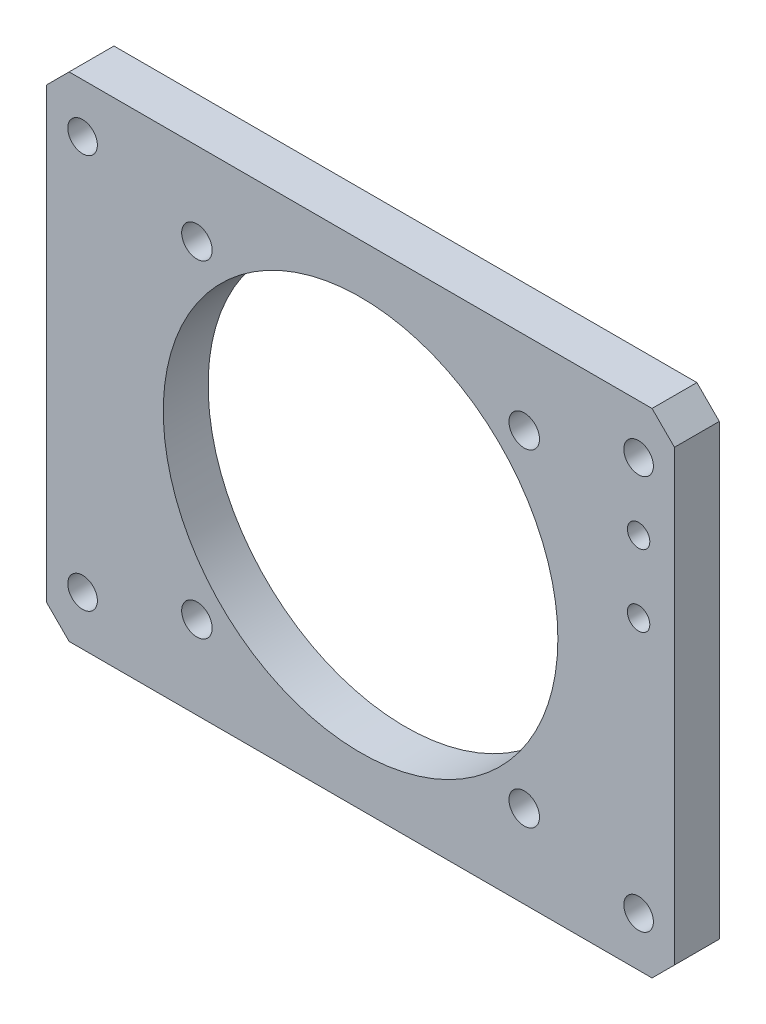
SolidWorks part; units mm, degrees
material "Q235-A"
ref_plane "Front Plane" through (0, 0, 0) normal (0, 0, 1) x (1, 0, 0)
ref_plane "Top Plane" through (0, 0, 0) normal (0, 1, 0) x (1, 0, 0)
ref_plane "Right Plane" through (0, 0, 0) normal (1, 0, 0) x (0, 0, -1)
sketch "Sketch1" plane through (0, 0, 0) normal (0, 0, 1) x (1, 0, 0)
  line L0 (5.5346, 71.5113) -> (5.5346, -38.4887) construction
  line L1 (-64.4654, 71.5113) -> (75.5346, 71.5113)
  line L2 (-64.4654, 71.5113) -> (-64.4654, -38.4887)
  line L3 (-64.4654, -38.4887) -> (75.5346, -38.4887)
  line L4 (75.5346, 71.5113) -> (75.5346, -38.4887)
  line L5 (-64.4654, 16.5113) -> (75.5346, 16.5113) construction
  line L7 (-56.4654, -27.4887) -> (67.5346, -27.4887) construction
  line L8 (-56.4654, -27.4887) -> (-56.4654, 60.5113) construction
  line L9 (-56.4654, 60.5113) -> (67.5346, 60.5113) construction
  line L10 (67.5346, -27.4887) -> (67.5346, 60.5113) construction
  line L11 (-56.4654, -27.4887) -> (67.5346, 60.5113) construction
  line L12 (-56.4654, 60.5113) -> (67.5346, -27.4887) construction
  circle A0 centre (5.5346, 16.5113) radius 44
  circle A1 centre (-56.4654, 60.5113) radius 3.3
  circle A2 centre (-56.4654, -27.4887) radius 3.3
  circle A3 centre (67.5346, -27.4887) radius 3.3
  circle A4 centre (67.5346, 60.5113) radius 3.3
  circle A5 centre (-56.4654, 60.5113) radius 3.3
  dimension "D3" = 124
  dimension "D1" = 140
  dimension "D2" = 110
  dimension "D4" = 88
extrude "Boss-Extrude1" add sketch "Sketch1" along normal blind 10 contours L4 L1 L2 L3 A4 A3 A2 A1 A0
sketch "Sketch2" plane through (0, 0, 10) normal (0, 0, 1) x (1, 0, 0)
  line L1 (-30.9654, -19.9887) -> (42.0346, -19.9887)
  line L2 (-30.9654, -19.9887) -> (-30.9654, 53.0113)
  line L3 (-30.9654, 53.0113) -> (42.0346, 53.0113)
  line L4 (42.0346, -19.9887) -> (42.0346, 53.0113)
  line L5 (-30.9654, -19.9887) -> (42.0346, 53.0113) construction
  line L6 (-30.9654, 53.0113) -> (42.0346, -19.9887) construction
  point P0 (5.5346, 16.5113)
  dimension "D1" = 73
  dimension "D2" = 73
hole_wizard "M8 Tapped Hole1" positions "Sketch3" profile "Sketch4" tap size "M8" standard "GB" end condition through all
sketch "Sketch3" plane through (0, 0, 10) normal (0, 0, 1) x (1, 0, 0)
  point P0 (-30.9654, 53.0113)
  point P3 (42.0346, 53.0113)
  point P6 (42.0346, -19.9887)
  point P9 (-30.9654, -19.9887)
sketch "Sketch4" plane through (-30.9654, 53.0113, 10) normal (1, 0, 0) x (0, -1, 0)
  line L0 (0, 0) -> (0, 10)
  line L1 (0, 10) -> (3.4, 10)
  line L2 (3.4, 10) -> (3.4, 0)
  line L5 (3.4, 0) -> (0, 0)
  line L11 (0, -6.35) -> (0, 107.95) construction
  dimension "通孔螺纹孔钻头直径" = 6.8
  dimension "通孔螺纹孔钻头深度" = 10
cosmetic thread "Cosmetic thread 1"
cosmetic thread "Cosmetic thread 2"
cosmetic thread "Cosmetic thread 3"
cosmetic thread "Cosmetic thread 4"
chamfer "Chamfer1" distance 5 angle 45 4 edges at (75.5346, -38.4887, 5) (75.5346, 71.5113, 5) (-64.4654, 71.5113, 5) (-64.4654, -38.4887, 5)
sketch "Sketch5" plane through (0, 0, 10) normal (0, 0, 1) x (1, 0, 0)
  line L0 (-59.4654, 71.5113) -> (70.5346, 71.5113) construction
  line L1 (-56.4654, -27.4887) -> (67.5346, -27.4887) construction
  line L2 (-56.4654, -27.4887) -> (-56.4654, 60.5113) construction
  line L3 (-56.4654, 60.5113) -> (67.5346, 60.5113) construction
  line L4 (67.5346, -27.4887) -> (67.5346, 60.5113) construction
  line L5 (-56.4654, -27.4887) -> (67.5346, 60.5113) construction
  line L6 (-56.4654, 60.5113) -> (67.5346, -27.4887) construction
  circle A0 centre (67.5346, 45.5113) radius 2.2296
  circle A1 centre (67.5346, 29.5113) radius 2.2296
  point P0 (5.5346, 16.5113)
  dimension "D1" = 26
  dimension "D2" = 16
hole_wizard "M6 Tapped Hole1" positions "Sketch6" profile "Sketch7" tap size "M6" standard "GB" end condition through all
sketch "Sketch6" plane through (0, 0, 10) normal (0, 0, 1) x (1, 0, 0)
  point P0 (67.5346, 45.5113)
  point P3 (67.5346, 29.5113)
sketch "Sketch7" plane through (67.5346, 45.5113, 10) normal (1, 0, 0) x (0, -1, 0)
  line L0 (0, 0) -> (0, 10)
  line L1 (0, 10) -> (2.5, 10)
  line L2 (2.5, 10) -> (2.5, 0)
  line L5 (2.5, 0) -> (0, 0)
  line L11 (0, -6.35) -> (0, 107.95) construction
  dimension "通孔螺纹孔钻头直径" = 5
  dimension "通孔螺纹孔钻头深度" = 10
cosmetic thread "Cosmetic thread 5"
cosmetic thread "Cosmetic thread 6"
